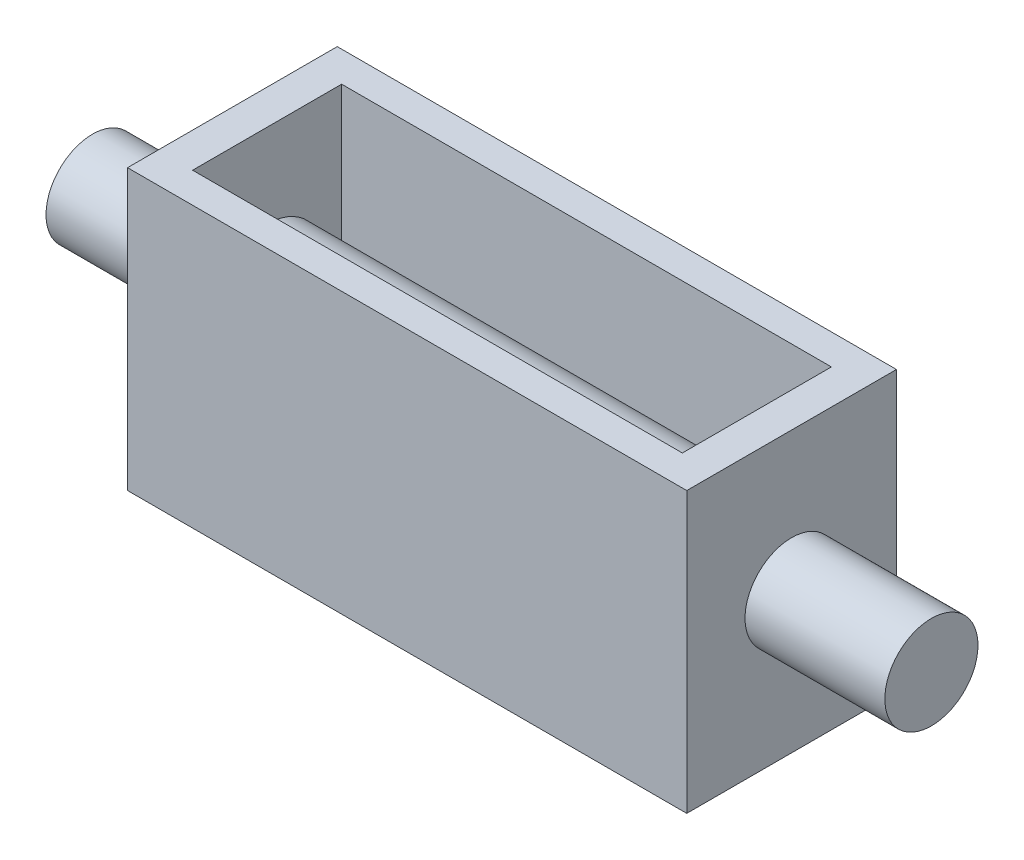
from build123d import *

# Parameters (mm, degrees)
SKETCH1_W           = 40
SKETCH1_H           = 15
BOSS_EXTRUDE1_DEPTH = 20
SKETCH2_W           = 35.032113562
SKETCH2_H           = 10.660333008
CUT_EXTRUDE1_DEPTH  = 10
SKETCH3_R           = 4
BOSS_EXTRUDE2_DEPTH = 35.032113562
SKETCH4_R           = 3.332307017
BOSS_EXTRUDE3_DEPTH = 10
BOSS_EXTRUDE4_START = 10
SKETCH5_R           = 3.332307017
BOSS_EXTRUDE4_DEPTH = 10
SCALE1_SCALE        = 0.7


with BuildPart() as part:
    # Sketch1 → Boss-Extrude1 (new body)
    with BuildSketch(Plane(origin=(0, 0, 0), x_dir=(1, 0, 0), z_dir=(0, 1, 0))):
        Rectangle(SKETCH1_W, SKETCH1_H)
    extrude(amount=BOSS_EXTRUDE1_DEPTH)

    # Sketch2 → Cut-Extrude1 (cut)
    with BuildSketch(Plane(origin=(0, 20, 0), x_dir=(1, 0, 0), z_dir=(0, 1, 0))):
        Rectangle(SKETCH2_W, SKETCH2_H)
    extrude(amount=-CUT_EXTRUDE1_DEPTH, mode=Mode.SUBTRACT)

    # Sketch3 → Boss-Extrude2 (add)
    with BuildSketch(Plane(origin=(-17.516056781, 0, 0), x_dir=(0, 0, -1), z_dir=(1, 0, 0))):
        with Locations((0, 10)):
            Circle(SKETCH3_R)
    extrude(amount=BOSS_EXTRUDE2_DEPTH)

    # Sketch4 → Boss-Extrude3 (add)
    with BuildSketch(Plane.ZY.offset(20)):
        with Locations((0, 10)):
            Circle(SKETCH4_R)
    extrude(amount=BOSS_EXTRUDE3_DEPTH)

    # Sketch5 → Boss-Extrude4 (add)
    with BuildSketch(Plane(origin=(20, 0, 0), x_dir=(0, 0, -1), z_dir=(1, 0, 0)).offset(BOSS_EXTRUDE4_START)):
        with Locations(Location((0, 10, 0), (0, 0, 180))):
            Circle(SKETCH5_R)
    extrude(amount=-BOSS_EXTRUDE4_DEPTH)


with BuildPart() as part_1:
    # Scale1: scaled about (0, 0, 0)
    add(part.part.scale(SCALE1_SCALE))


solid = part_1.part
